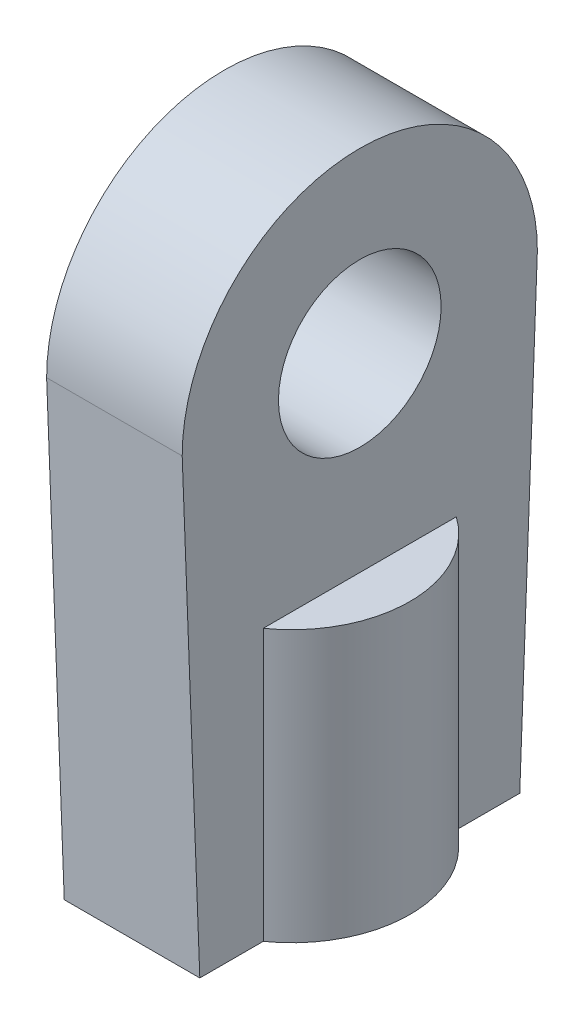
from build123d import *

# Parameters (mm, degrees)
SKETCH1_R           = 30
BOSS_EXTRUDE1_DEPTH = 25
SKETCH2_R           = 43.5
BOSS_EXTRUDE2_DEPTH = 100


with BuildPart() as part:
    # Sketch1 → Boss-Extrude1 (new, symmetric)
    with BuildSketch(Plane(origin=(0, 0, 0), x_dir=(0, 0, -1), z_dir=(1, 0, 0))):
        with BuildLine():
            Line((-65.5, 170), (-59, 0))
            Line((-59, 0), (59, 0))
            Line((59, 0), (65.5, 170))
            ThreePointArc((65.5, 170), (0, 235.5), (-65.5, 170))
        make_face()
        with Locations((0, 170)):
            Circle(SKETCH1_R, mode=Mode.SUBTRACT)
    extrude(amount=BOSS_EXTRUDE1_DEPTH, both=True)

    # Sketch2 → Boss-Extrude2 (add)
    with BuildSketch(Plane(origin=(0, 0, 0), x_dir=(1, 0, 0), z_dir=(0, 1, 0))):
        Circle(SKETCH2_R)
    extrude(amount=BOSS_EXTRUDE2_DEPTH)


solid = part.part
